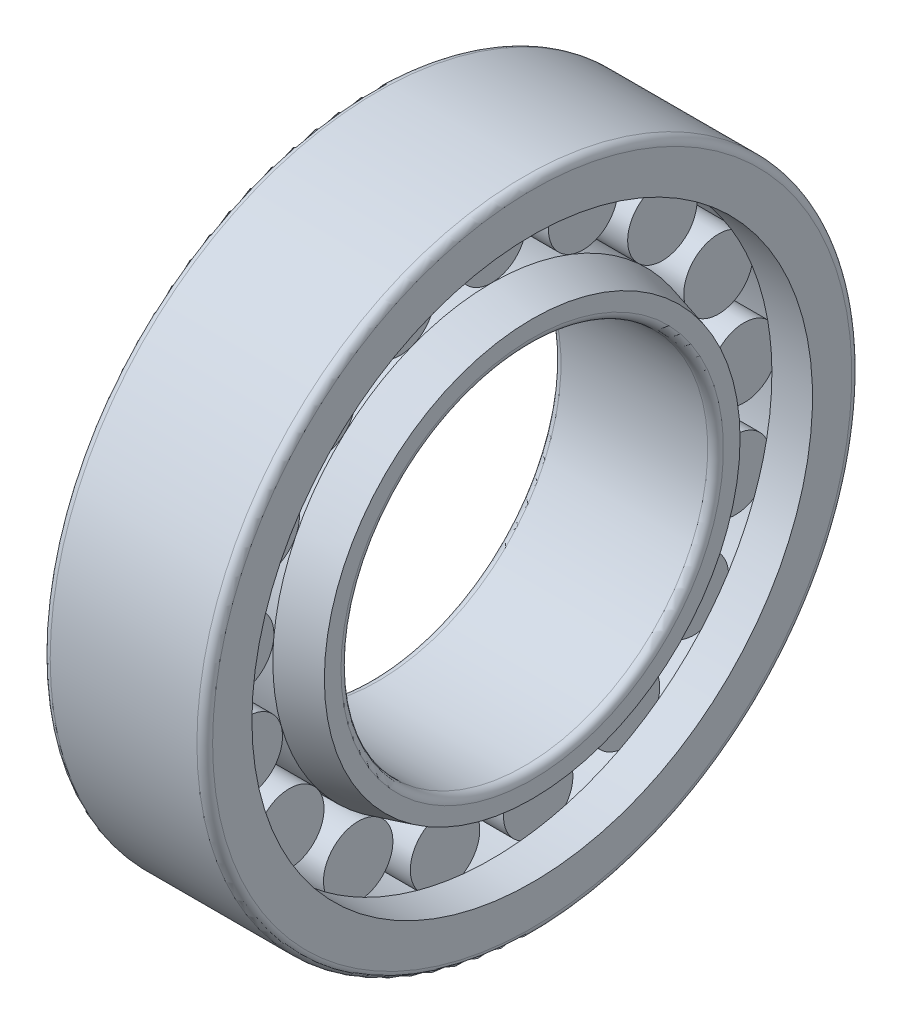
SolidWorks part; units mm, degrees
revolve "Base-Revolve" add sketch "Sketch2" angle 360 about L0
sketch "Sketch2" plane through (0, 0, 0) normal (0, 0, 1) x (1, 0, 0)
  line L0 (-10.0801, 0) -> (21.9267, 0) construction
  line L1 (7.75, 41.75) -> (23.25, 41.75)
  line L2 (0, 37.3831) -> (7.75, 41.75)
  line L3 (0, 37.3831) -> (0, 36.5)
  line L4 (1.5, 35) -> (29.5, 35)
  line L5 (31, 39.6734) -> (31, 36.5)
  line L7 (31, 39.6734) -> (23.25, 41.75)
  arc A0 (29.5, 35) -> (31, 36.5) centre (29.5, 36.5) ccw
  arc A1 (0, 36.5) -> (1.5, 35) centre (1.5, 36.5) ccw
  point P13 (31, 35)
  point P16 (0, 35)
material "GCr15SiMn"
ref_plane "Plane1" through (0, 0, 0) normal (0, 0, 1) x (1, 0, 0)
ref_plane "Plane2" through (0, 0, 0) normal (0, 1, 0) x (1, 0, 0)
ref_plane "Plane3" through (0, 0, 0) normal (1, 0, 0) x (0, 0, -1)
sketch "Sketch dimensions" plane through (0, 0, 0) normal (0, 0, 1) x (1, 0, 0)
  line L0 (0, 0) -> (1.5, 0)
  line L1 (1.5, 0) -> (3, 0)
  line L2 (3, 0) -> (34, 0)
  line L3 (34, 0) -> (104, 0)
  line L4 (104, 0) -> (187.5, 0)
  line L5 (187.5, 0) -> (312.5, 0)
  line L7 (312.5, 0) -> (422.5, 0)
sketch "Sketch3" plane through (0, 0, 0) normal (0, 0, 1) x (1, 0, 0)
  line L0 (7.75, 41.75) -> (7.75, -41.75) construction
  line L1 (23.25, 41.75) -> (23.25, -41.75) construction
  line L2 (-1.6039, 48.375) -> (13.5036, 48.375) construction
  line L4 (7.75, 48.375) -> (23.25, 48.375)
  line L5 (7.75, 48.375) -> (7.75, 41.7499)
  line L6 (7.75, 41.7499) -> (23.25, 41.7499)
  line L7 (23.25, 48.375) -> (23.25, 41.7499)
revolve "Boss-Revolve1" add sketch "Sketch3" angle 360 about L2
sketch "Sketch4" plane through (0, 0, 0) normal (0, 0, 1) x (1, 0, 0)
  line L0 (0, 0) -> (17.8006, 0) construction
  line L1 (-10.0801, 0) -> (21.9267, 0) construction
  line L2 (23.25, 53.5) -> (31, 53.5)
  line L3 (1.5, 62.5) -> (29.5, 62.5)
  line L4 (0, 61) -> (0, 53.5)
  line L5 (0, 53.5) -> (7.75, 53.5)
  line L6 (31, 61) -> (31, 53.5)
  line L7 (7.75, 55) -> (23.25, 55)
  line L8 (7.75, 55) -> (7.75, 53.5)
  line L10 (23.25, 55) -> (23.25, 53.5)
  arc A0 (29.5, 62.5) -> (31, 61) centre (29.5, 61) cw
  arc A1 (1.5, 62.5) -> (0, 61) centre (1.5, 61) ccw
  point P15 (31, 62.5)
  point P18 (0, 62.5)
revolve "Boss-Revolve2" add sketch "Sketch4" angle 360 about L0
pattern_circular "CirPattern1" count 17 over 360 about axis through (0, 0, 0) along (1, 0, 0) of "Boss-Revolve1"
equation "\"DD@Sketch2\" = \"内径@Sketch dimensions\""
equation "\"FW@Sketch2\" = \"参考FW@Sketch dimensions\""
equation "\"D1@Sketch2\" = \"倒角小@Sketch dimensions\""
equation "\"EW@Sketch4\" = \"参考EW@Sketch dimensions\""
equation "\"D@Sketch4\" = \"外径@Sketch dimensions\""
equation "\"D2@Sketch4\" = \"倒角大@Sketch dimensions\""
equation "\"B@Sketch4\" = \"宽度@Sketch dimensions\""
equation "\"D1@Sketch3\" =  ( \"EW@Sketch4\" - \"FW@Sketch2\" )  / 4 + \"FW@Sketch2\" / 2"
equation "\"D2@Sketch3\" =  0.25*( \"EW@Sketch4\" - \"FW@Sketch2\" ) +0.0001"
equation "\"D2@Sketch2\" = \"B@Sketch4\""
equation "\"D4@Sketch2\" = \"FW@Sketch2\" + 4 *\"D1@Sketch2\""
equation "\"滚珠位置@Sketch2\" = \"D2@Sketch2\"/4"
equation "\"D3@Sketch4\" = \"D2@Sketch4\""
equation "\"D1@CirPattern1\" = 0.75*\"D1@Sketch3\" * 3.14 / \"D2@Sketch3\""
